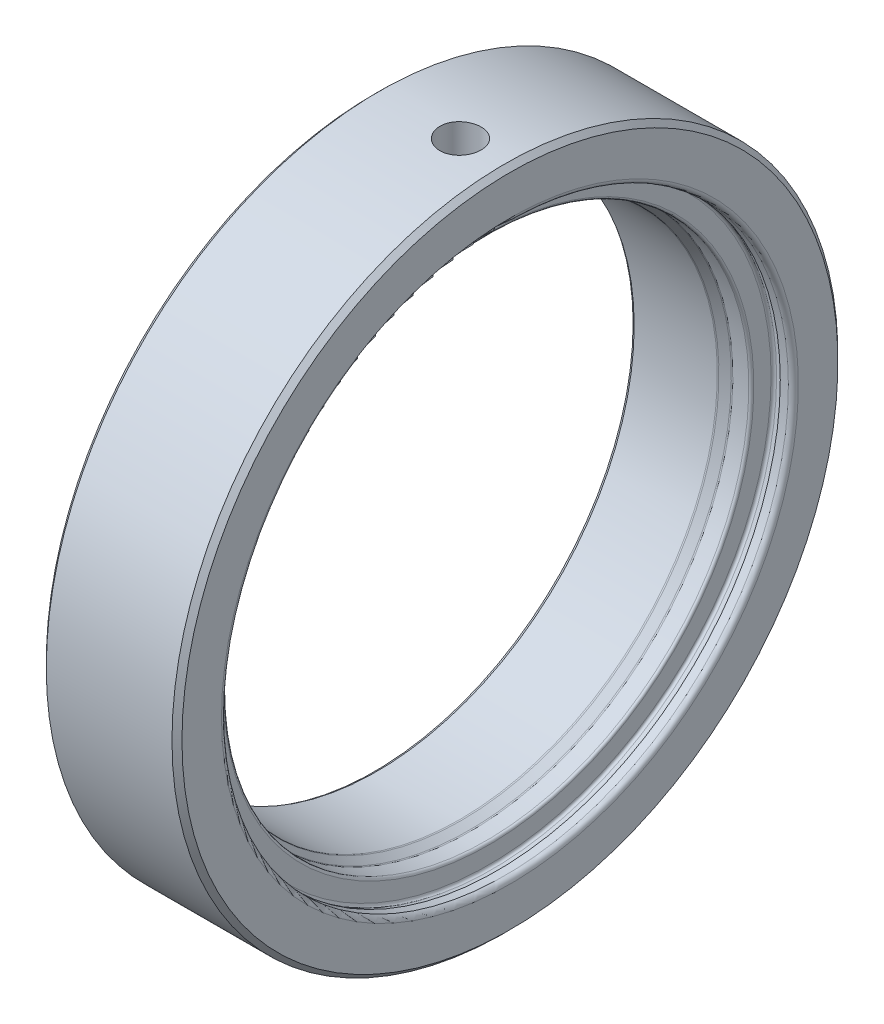
SolidWorks part; units mm, degrees
material "45"
ref_plane "Front plane" through (0, 0, 0) normal (0, 0, 1) x (1, 0, 0)
ref_plane "Top plane" through (0, 0, 0) normal (0, 1, 0) x (1, 0, 0)
ref_plane "Right plane" through (0, 0, 0) normal (1, 0, 0) x (0, 0, -1)
sketch "Sketch1" plane through (0, 0, 0) normal (0, 0, 1) x (1, 0, 0)
  line L0 (-48.0801, 0) -> (53.6066, 0) construction
  line L1 (0, 58.5804) -> (0, -55.2645) construction
  line L2 (0, 101.6) -> (41.402, 101.6)
  line L3 (41.402, 101.6) -> (41.402, 88.011)
  line L4 (39.878, 86.487) -> (37.4009, 86.487)
  line L5 (34.925, 80.899) -> (34.925, 86.1574)
  line L6 (34.163, 80.137) -> (29.2936, 80.137)
  line L7 (28.9126, 80.0349) -> (26.5166, 78.6516)
  line L8 (26.1356, 78.5495) -> (0, 78.5495)
  line L9 (0, 78.5495) -> (0, 101.6)
  line L10 (35.8842, 86.8934) -> (37.4009, 86.487)
  arc A0 (35.8842, 86.8934) -> (34.925, 86.1574) centre (35.687, 86.1574) ccw
  arc A1 (41.402, 88.011) -> (39.878, 86.487) centre (39.878, 88.011) cw
  arc A2 (26.5166, 78.6516) -> (26.1356, 78.5495) centre (26.1356, 79.3115) cw
  arc A3 (29.2936, 80.137) -> (28.9126, 80.0349) centre (29.2936, 79.375) ccw
  arc A4 (34.925, 80.899) -> (34.163, 80.137) centre (34.163, 80.899) cw
  point P20 (26.3398, 78.5495)
  point P23 (29.0894, 80.137)
  dimension "D10" = 0.762
  dimension "D12" = 1.524
  dimension "D14" = 0.762
  dimension "D15" = 0.762
  dimension "D16" = 0.762
  dimension "D1" = 203.2
  dimension "D2" = 172.974
  dimension "D3" = 160.274
  dimension "D4" = 157.099
  dimension "D5" = 41.402
  dimension "D6" = 6.477
  dimension "D7" = 15.0622
  dimension "D8" = 12.3126
  dimension "D9" = 15
  dimension "D11" = 0.4064
  dimension "D13" = 30
revolve "Revolve1" add sketch "Sketch1" angle 360 about L0
chamfer "Chamfer2" distance 0.762 angle 30 1 edges at (0, 0, 78.5495)
chamfer "Chamfer3" distance 1.524 angle 45 2 edges at (41.402, 0, 101.6) (0, 0, 101.6)
ref_plane "Plane1" through (20.701, 101.6, 0) normal (0, 1, 0) x (0, 0, -1)
sketch "Sketch2" plane through (20.701, 101.6, 0) normal (0, 1, 0) x (0, 0, -1)
  line L0 (-100.076, -20.701) -> (100.076, -20.701) construction
  line L1 (0, 6.2988) -> (0, -11.6294) construction
  point P0 (0, -5.6134)
  dimension "D1" = 15.0876
hole_wizard "1/8 NPT Tapped Hole1" positions "3DSketch1" profile "Sketch3" size "1/8" standard "Ansi Inch"
sketch3d "3DSketch1"
  point P0 (26.3144, 101.6, 0)
  point P3 (26.3144, 101.6, 0)
  point P8 (26.3144, 101.6, 0)
cosmetic thread "Hole Thread2" parameters "D1"=58.42, "D2"=13.3707
sketch "Sketch3" plane through (26.3144, 101.6, 0) normal (1, 0, 0) x (0, 0, 1)
  line L0 (0, 0) -> (0, 65.6525)
  line L1 (4.2164, 63.119) -> (0, 65.6525)
  line L2 (-4.2164, 63.119) -> (0, 65.6525) construction
  line L3 (4.2164, 63.119) -> (4.2164, 58.42)
  line L4 (4.2164, 58.42) -> (6.2866, 58.42)
  line L5 (6.2866, 58.42) -> (6.2866, 0)
  line L6 (-6.2866, 58.42) -> (-6.2866, 0) construction
  line L7 (6.2866, 0) -> (0, 0)
  line L8 (0, -6.35) -> (0, 107.95) construction
  line L11 (-4.2164, 58.42) -> (-6.2866, 58.42) construction
  dimension "蹟恇謂郰芛眻噤" = 8.4328
  dimension "蹟恇謂郰芛旮僅" = 63.119
  dimension "蹟恇眻噤" = 12.5732
  dimension "蹟恇褒僅" = 0
  dimension "蹟恇旮僅" = 58.42
  dimension "絳芛褒僅" = 118
